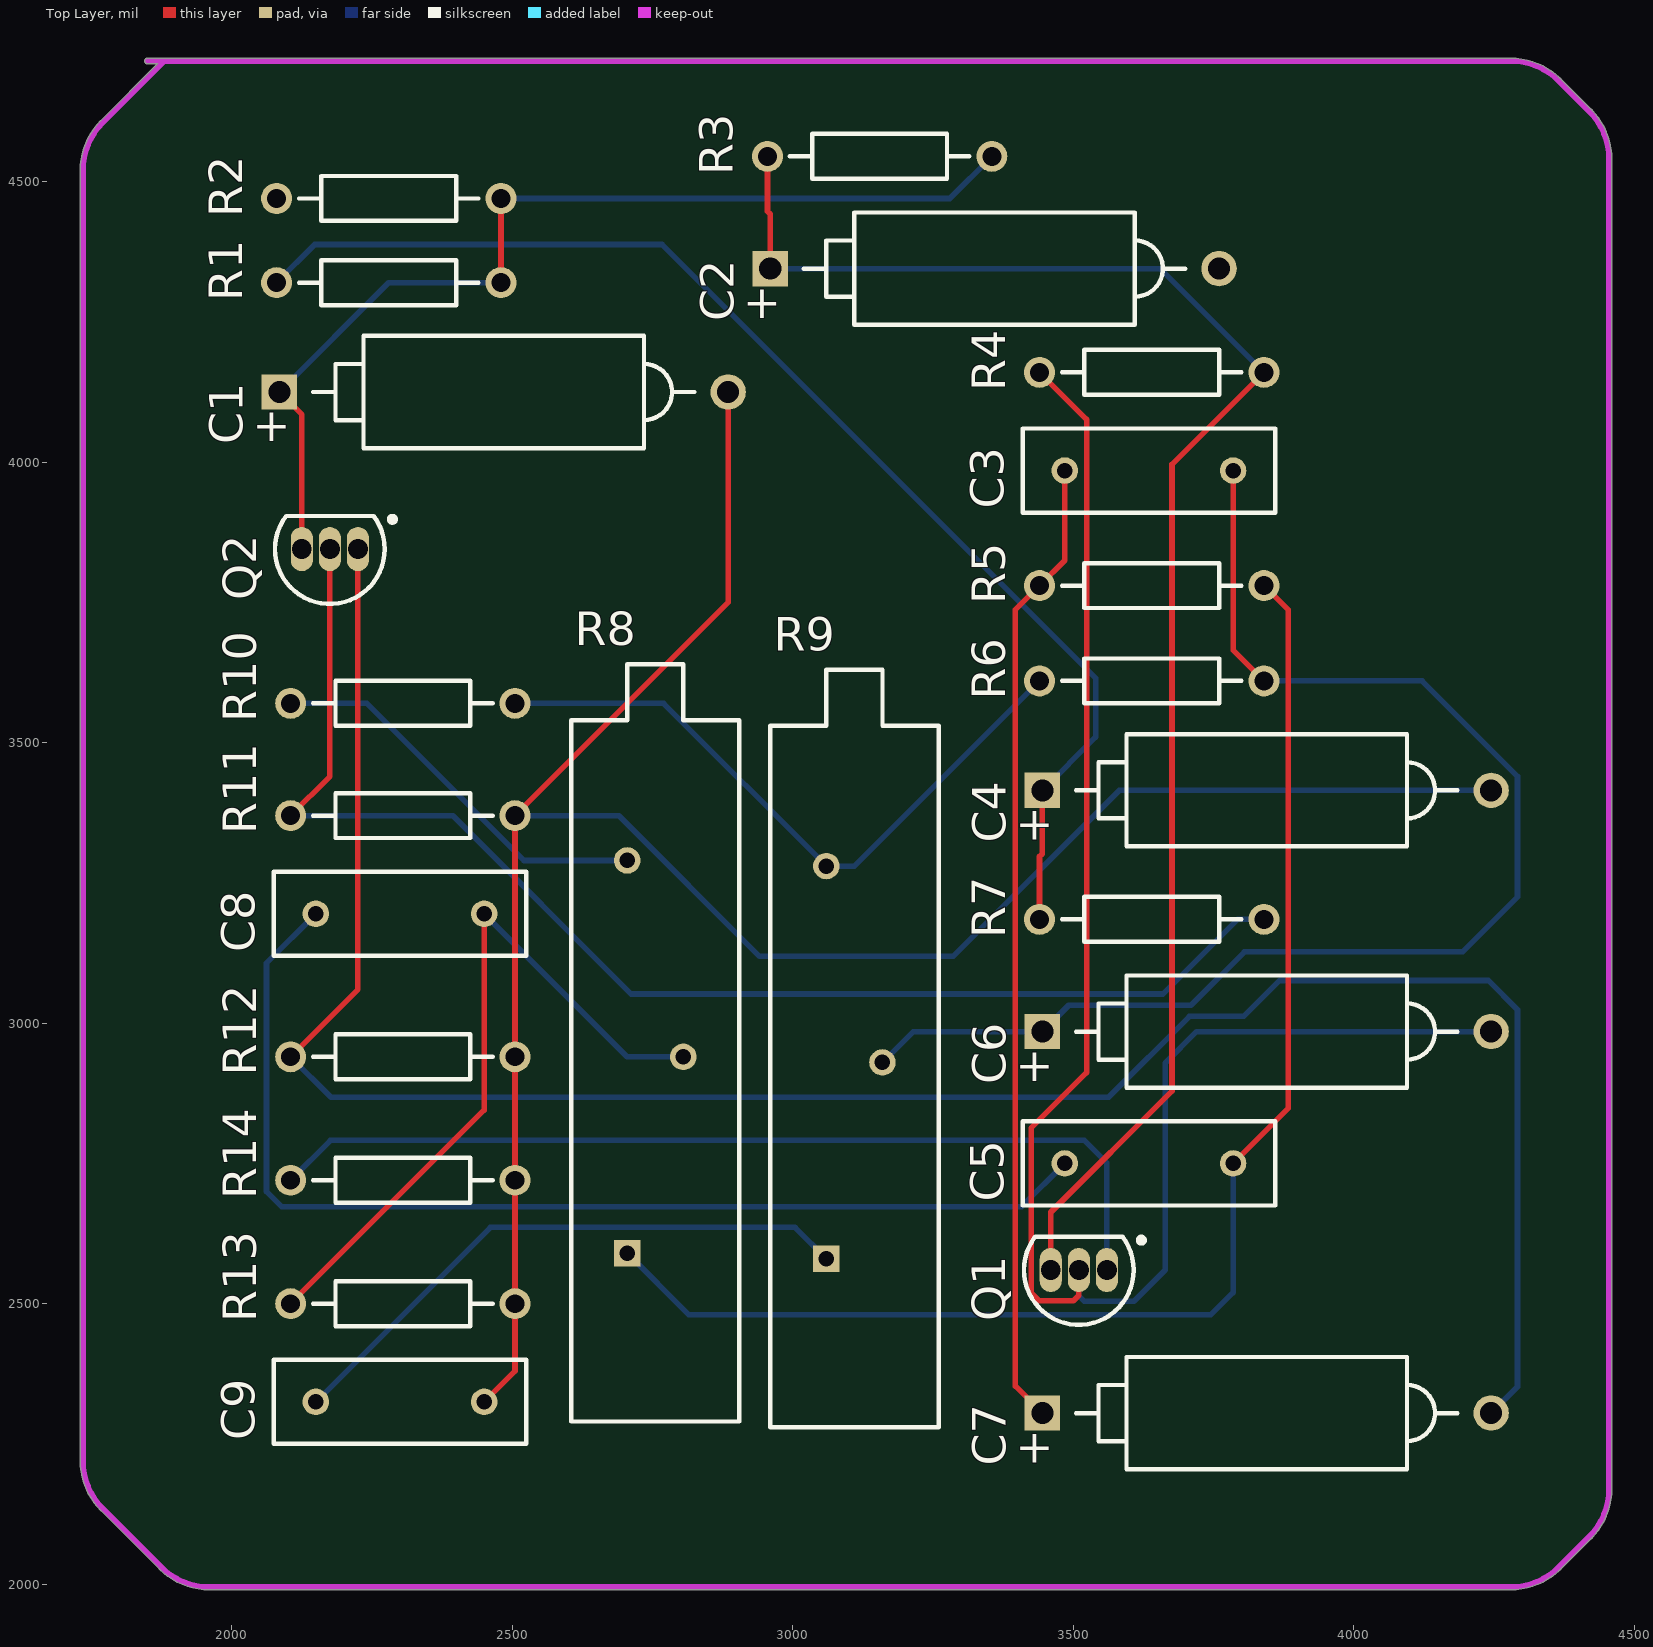
[diagram p0: Top Layer view]
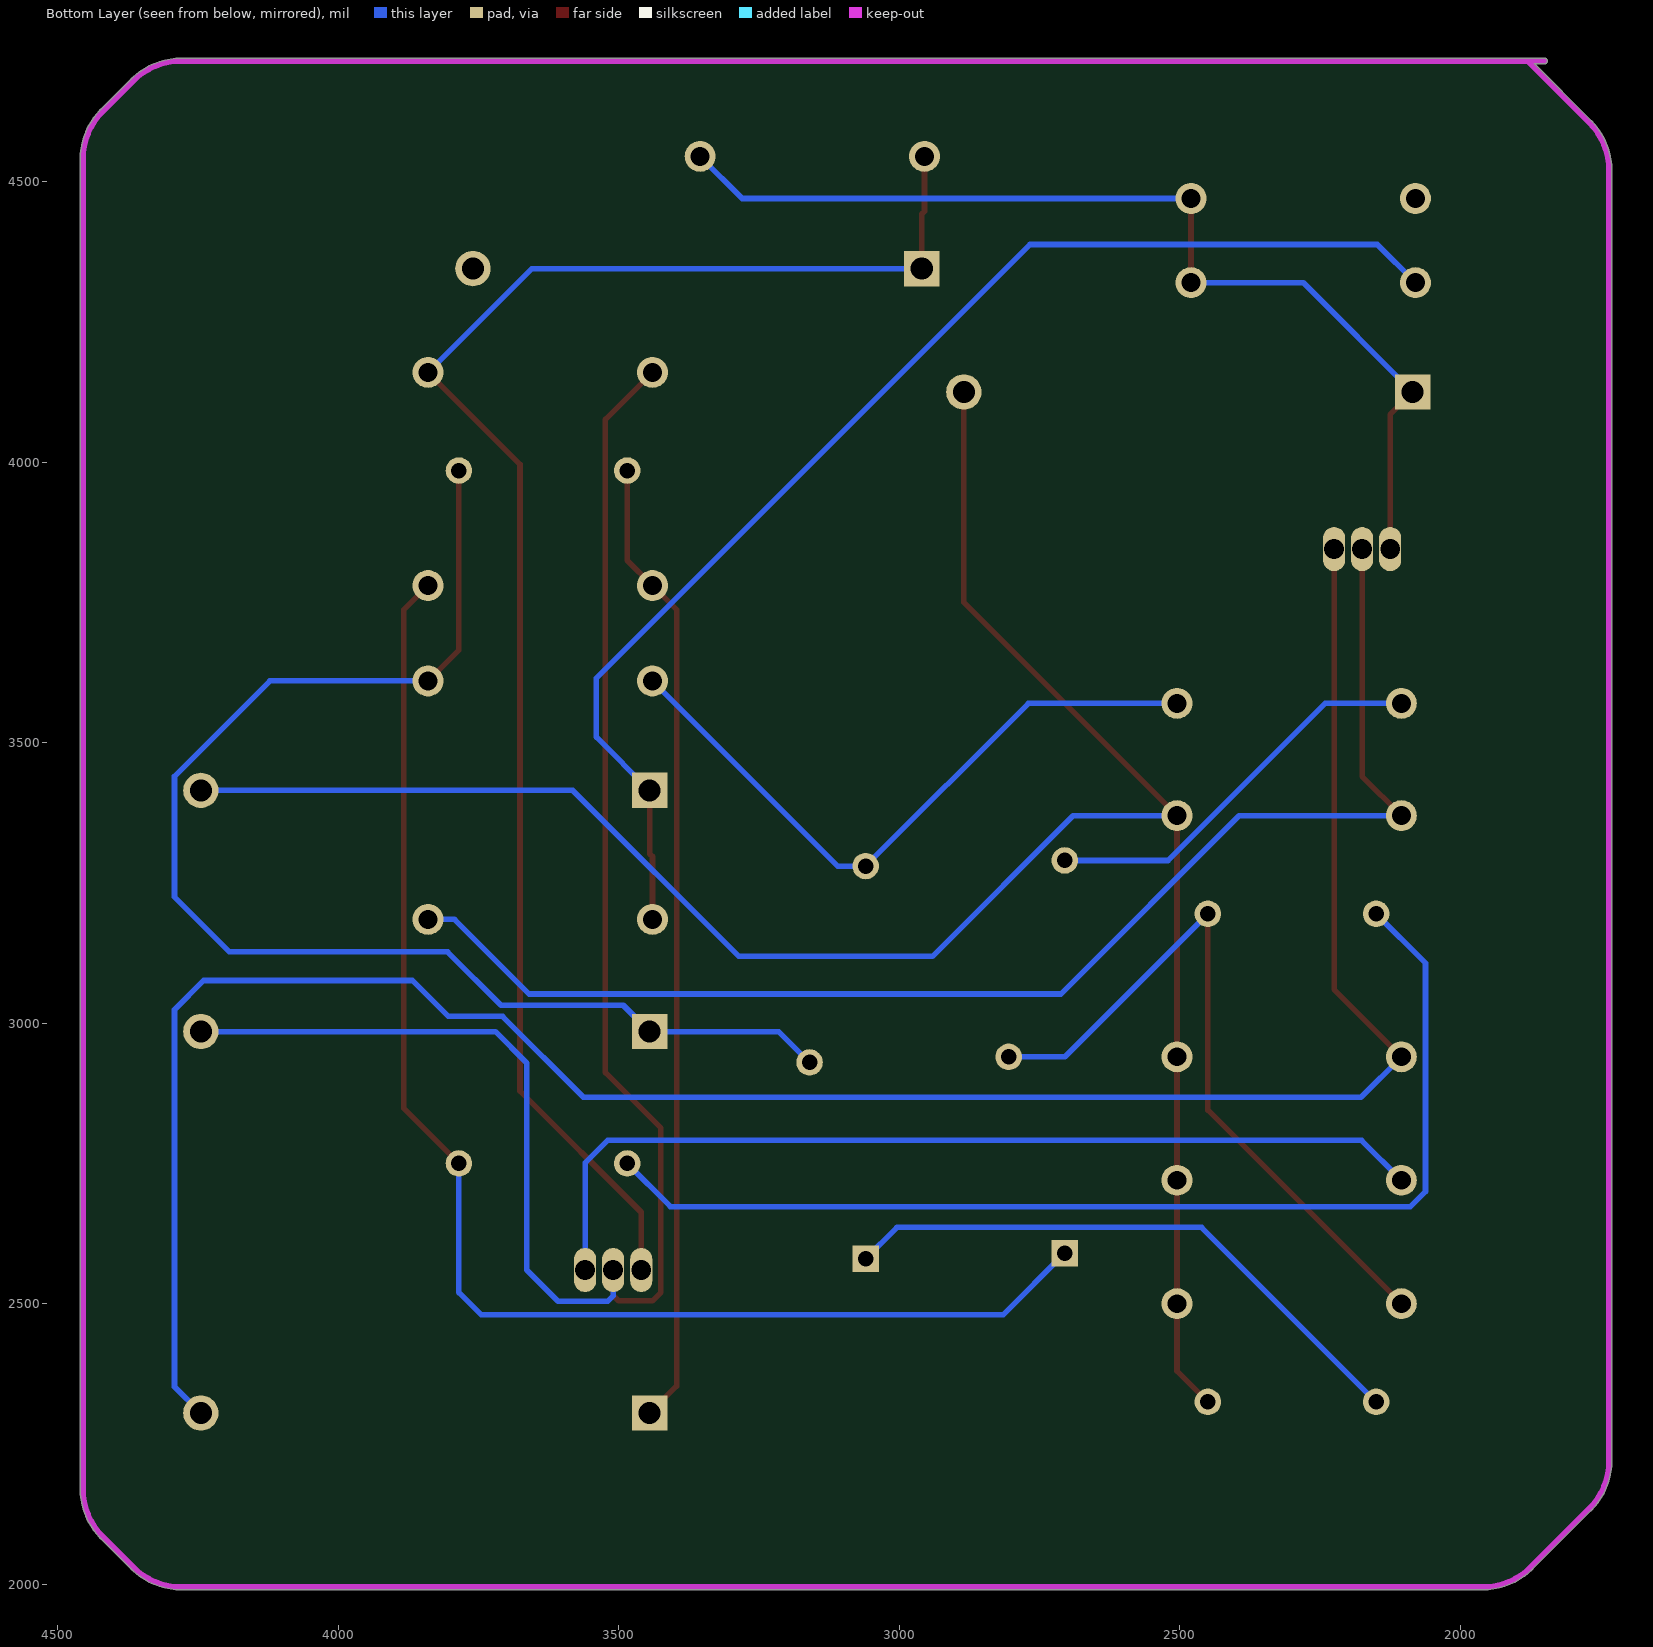
[diagram p1: Bottom Layer view, seen from below]
# Altium PCB MISC80684.PcbDoc
Units mil, origin at the board's own origin, x right, y up, seen from the top; angles counter-clockwise.
Board outline 2730.03 x 2730.03 mil, 2 copper layers (Top Layer, Bottom Layer); 25 components, 17 nets, 54 pads, 0 vias.

## Layer stack, top to bottom (the 12.6 mil dielectric is the usual default, probably not edited)
Top Solder: solder mask 0.4, Solder Resist, Dk 3.5
Top Layer: signal copper 1.4
Dielectric 1: dielectric 12.6, FR-4, Dk 4.8
Bottom Layer: signal copper 1.4
Bottom Solder: solder mask 0.4, Solder Resist, Dk 3.5

## Board outline
1766.83,2131.08 cw(c1770.36,2134.64) 1766.81,2131.1 1871.1,2026.81 cw(c1874.64,2030.36) 1871.08,2026.83 1871.1,2026.81 ccw(c1960,2115.71) 1960,1989.98 4280,1989.98 ccw(c4280,2115.71) 4368.9,2026.81 4423.19,2081.1 ccw(c4334.29,2170) 4460.02,2170 4460.02,4540 ccw(c4334.29,4540) 4423.19,4628.9 4368.9,4683.19 cw(c4365.36,4679.64) 4368.92,4683.17 4368.9,4683.19 ccw(c4280,4594.29) 4280,4720.02 1850,4720.02 ccw(c1850,4715) 1850,4709.98 1867.89,4709.98 1766.81,4608.9 cw(c1770.36,4605.36) 1766.83,4608.92 1766.81,4608.9 ccw(c1855.71,4520) 1729.98,4520 1729.98,2220 ccw(c1855.71,2220)

## Design rules (kind name [scope] priority, off if disabled: settings)
Clearance [All] p1: gap=10
PolygonConnect [All] p1: connectstyle=Relief reliefconductorwidth=10 reliefentries=4 polygonreliefangle="90 Angle" airgapwidth=10
RoutingVias [All] p1: holewidth=28 width=50 viastyle="Through Hole" minholewidth=28 minwidth=50 maxholewidth=28 maxwidth=50
SolderMaskExpansion [All] p1: expansion=4
Width [All] p1: maxlimit=10 minlimit=10 preferedwidth=10
30 further rules are at their usual default settings.

## Components (designator, comment, footprint, x,y, rotation, side; value= is the part's Value field where it differs from the comment)
C1 "Cap Pol2" POLAR0.8 2485,4125 r180 top
C2 "Cap Pol2" POLAR0.8 3360,4345 r180 top
C3 "Cap" RAD-0.3 3635,3985 r180 top
C4 "Cap Pol2" POLAR0.8 3845,3415 r180 top
C5 "Cap" RAD-0.3 3635,2750 r180 top
C6 "Cap Pol2" POLAR0.8 3845,2985 r180 top
C7 "Cap Pol2" POLAR0.8 3845,2305 r180 top
C8 "Cap" RAD-0.3 2300,3195 r180 top
C9 "Cap" RAD-0.3 2300,2325 r180 top
Q1 "2N3904" TO-92A 3510,2560 r90 top
Q2 "2N3904" TO-92A 2175,3845 r90 top
R1 "Res2" AXIAL-0.4 2280,4320 r180 top
R2 "Res2" AXIAL-0.4 2280,4470 r180 top
R3 "Res2" AXIAL-0.4 3155,4545 r180 top
R4 "Res2" AXIAL-0.4 3640,4160 r180 top
R5 "Res2" AXIAL-0.4 3640,3780 r180 top
R6 "Res2" AXIAL-0.4 3640,3610 r180 top
R7 "Res2" AXIAL-0.4 3640,3185 r180 top
R8 "Res Tap" VR3 2755,2940 r90 top
R9 "Res Tap" VR3 3110,2930 r90 top
R10 "Res2" AXIAL-0.4 2305,3570 r180 top
R11 "Res2" AXIAL-0.4 2305,3370 r180 top
R12 "Res2" AXIAL-0.4 2305,2940 r180 top
R13 "Res2" AXIAL-0.4 2305,2500 r180 top
R14 "Res2" AXIAL-0.4 2305,2720 r180 top

## Footprints (in the part's own frame and the unit in brackets; to place one, negate y for a bottom-side part, rotate by r counter-clockwise, add the part's x,y. Pads: shape width x height; smd on the part's side, far side on the other; paste and mask are expansions set on the pad)
AXIAL-0.4 [mm] "Axial Device, Thru-Hole; 2 Leads; 0.4 in Pin Spacing"
  round 1.4 hole 0.85: 1(-5.08,0) 2(5.08,0)
  silkscreen extent -4.06,-1.02 4.06,1.02
POLAR0.8 [mm] "Polarized Capacitor; 2 Leads"
  rect 1.6x1.6 hole 1: 1(10.16,0)
  round 1.6 hole 1: 2(-10.16,0)
  silkscreen extent -8.64,-2.54 8.64,2.54
RAD-0.3 [mm] "Radial Cap, Thru-Hole; 2 Leads; 0.3 in Pin Spacing"
  round 1.2 hole 0.7: 1(-3.81,0) 2(3.81,0)
  silkscreen extent -5.71,-1.91 5.71,1.91
TO-92A [mm] "TO, Flat Index; 3 In-Line, Axial Leads; Body Dia. 4.5mm; Leads 0.51 x 0.48 mm (max)"
  oval 2x1 hole 0.9: 1(0,-1.27) 2(0,0) 3(0,1.27)
  silkscreen extent -2.48,-2.96 1.5,2.48, body extent -2.48,-2.5 1.5,2.5, height 6.86
VR3 [mm] "Thru-Hole; 3 Leads"
  rect 1.2x1.2 hole 0.7: 1(-8.89,1.27)
  round 1.2 hole 0.7: 2(0,-1.27) 3(8.89,1.27)
  silkscreen extent -16.51,-3.81 17.78,3.81

## Part data
C1 C2 C4 C6 C7: "Polarized Capacitor (Axial)"
C3 C5 C8 C9: "Capacitor"
Q1 Q2: "NPN General Purpose Amplifier"
R1 R2 R3 R4 R5 R6 R7 R10 R11 R12 R13 R14: "Resistor"
R8 R9: "Tapped Resistor"

## Nets (pads, with @x,y where several pads share a name; then routed paths per layer and width w, separated by ;. In a path a pad name is that pad's centre, name@x,y a point inside that pad or via, vN(x,y) a via of type N, cw(c..) or ccw(c..) an arc to the next point about the centre after c; other vN are vias at no path point)
GND: C1.2 C4.2 C9.1 R11.1 R12.1 R13.1 R14.1 | length 3946.8
  Top Layer w10: C9.1 2505,2380 R13.1 R14.1 R12.1 R11.1 2885,3750 C1.2
  Bottom Layer w10: R11.1 2690,3370 2941,3119 3286,3119 3582,3415 C4.2
NetC1_1: C1.1 Q2.3 R1.1 R2.1 R3.1 | length 1828.4
  Top Layer w10: C1.1 2125,4085 Q2.3 ; R1.1 R2.1
  Bottom Layer w10: C1.1 2280,4320 R1.1 ; R2.1 3280,4470 R3.1
NetC2_1: C2.1 Q1.3 R3.2 R4.1 | length 2916.1
  Top Layer w10: R3.2 2955,4447 2960,4442 C2.1 ; Q1.3 3460,2663 3676,2879 3676,3996 R4.1
  Bottom Layer w10: C2.1 3655,4345 R4.1
NetC3_1: C3.1 C6.1 R6.1 R9.2 | length 2389.4
  Top Layer w10: C3.1 3785,3665 R6.1
  Bottom Layer w10: R9.2 3215,2985 C6.1 3492,3032 3710,3032 3805,3127 4194,3127 4292,3225 4292,3440 4122,3610 R6.1
NetC3_2: C3.2 C7.1 R5.2 | length 1736.3
  Top Layer w10: C7.1 3397,2353 3397,3737 R5.2 3485,3825 C3.2
NetC4_1: C4.1 R1.2 R7.2 | length 2279.8
  Top Layer w10: R7.2 3440,3297 3445,3302 C4.1
  Bottom Layer w10: R1.2 2148,4388 2767,4388 3540,3615 3540,3510 C4.1
NetC5_1: C5.1 R5.1 R8.1 | length 2460.5
  Top Layer w10: C5.1 3883,2848 3883,3737 R5.1
  Bottom Layer w10: R8.1 2815,2480 3745,2480 3785,2520 C5.1
NetC5_2: C5.2 C8.2 | length 1997.5
  Bottom Layer w10: C8.2 2062,3107 2062,2700 2089,2673 3408,2673 C5.2
NetC6_2: C6.2 Q1.2 R4.2 | length 3056.7
  Top Layer w10: R4.2 3524,4076 3524,2912 3425,2813 3425,2520 3440,2505 3500,2505 3510,2515 Q1.2
  Bottom Layer w10: Q1.2 3510,2514 3520,2504 3608,2504 3664,2560 3664,2929 3720,2985 C6.2
NetC7_2: C7.2 Q2.1 R12.2 | length 4017.7
  Top Layer w10: R12.2 2225,3060 Q2.1
  Bottom Layer w10: R12.2 2177,2868 3563,2868 3707,3012 3803.85,3012 3867.85,3076 4240,3076 4292,3024 4292,2352 C7.2
NetC8_1: C8.1 R8.2 R13.2 | length 1298.5
  Top Layer w10: R13.2 2450,2845 C8.1
  Bottom Layer w10: C8.1 2705,2940 R8.2
NetC9_2: C9.2 R9.1 | length 1062
  Bottom Layer w10: C9.2 2461,2636 3004,2636 R9.1
NetQ1_1: Q1.1 R14.2 | length 1692
  Bottom Layer w10: R14.2 2176,2791 3520,2791 3560,2751 Q1.1
NetQ2_2: Q2.2 R7.1 R11.2 | length 2425.8
  Top Layer w10: R11.2 2175,3440 Q2.2
  Bottom Layer w10: R11.2 2394.11,3370 2712.11,3052 3659.81,3052 3792.81,3185 R7.1
NetR6_2: R6.2 R9.3 R10.1 | length 1191.8
  Bottom Layer w10: R10.1 2770,3570 R9.3 3110,3280 R6.2
NetR8_3: R8.3 R10.2 | length 716
  Bottom Layer w10: R10.2 2241,3570 2521,3290 R8.3
VCC: R2.2
pads on no net: C2.2

## Keep-outs
Keep-Out Layer:
  lines w10: 1850,4715 4280,4715 cw(c4280,4594.29) 4365.36,4679.64 4419.64,4625.36 cw(c4334.29,4540) 4455,4540 4455,2170 cw(c4334.29,2170) 4419.64,2084.64 4365.36,2030.36 cw(c4280,2115.71) 4280,1995 1960,1995 cw(c1960,2115.71) 1874.64,2030.36 1770.36,2134.64 cw(c1855.71,2220) 1735,2220 1735,4520 cw(c1855.71,4520) 1770.36,4605.36 1880,4715